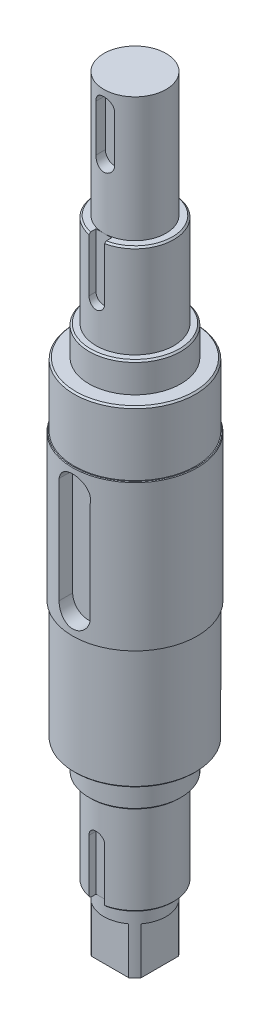
SolidWorks part; units mm, degrees
material "1045"
ref_plane "Front Plane" through (0, 0, 0) normal (0, 0, 1) x (1, 0, 0)
ref_plane "Top Plane" through (0, 0, 0) normal (0, 1, 0) x (1, 0, 0)
ref_plane "Right Plane" through (0, 0, 0) normal (1, 0, 0) x (0, 0, -1)
sketch "Sketch1" plane through (0, 0, 0) normal (0, 1, 0) x (1, 0, 0)
  circle A0 centre (0, 0) radius 20
  dimension "D1" = 40
extrude "Extrude1" add sketch "Sketch1" along normal blind 32 and the other way blind 15
sketch "草图1" plane through (0, -15, 0) normal (0, -1, 0) x (1, 0, 0)
  circle A0 centre (0, 0) radius 19.5
  dimension "D1" = 39
extrude "拉伸1" add sketch "草图1" along normal blind 38.5
sketch "Sketch2" plane through (0, 32, 0) normal (0, 1, 0) x (1, 0, 0)
  circle A0 centre (0, 0) radius 19.5
  dimension "D1" = 39
extrude "Extrude2" add sketch "Sketch2" along normal blind 20.5
ref_plane "Plane1" through (0, 0, 20) normal (0, 0, 1) x (1, 0, 0)
chamfer "Chamfer1" distance 0.2 angle 45 1 edges at (0, 32, 20)
sketch "Sketch4" plane through (0, 0, 20) normal (0, 0, 1) x (1, 0, 0)
  line L0 (0, 32) -> (0, -15) construction
  line L1 (19.8, 32) -> (-19.8, 32) construction
  line L2 (-19.5, -15) -> (19.5, -15) construction
  line L4 (-5, 26) -> (-5, -8)
  line L5 (5, 24) -> (5, -8)
  arc A0 (-5, 26) -> (5, 24) centre (0, 25) cw
  arc A1 (-5, -8) -> (5, -8) centre (0, -8) ccw
  dimension "D1" = 7
  dimension "D2" = 10
extrude "Cut-Extrude1" cut sketch "Sketch4" against normal blind 5
sketch "Sketch5" plane through (0, 52.5, 0) normal (0, 1, 0) x (1, 0, 0)
  circle A0 centre (0, 0) radius 14.75
  dimension "D1" = 29.5
extrude "Extrude3" add sketch "Sketch5" along normal blind 9.5
sketch "Sketch6" plane through (0, 62, 0) normal (0, 1, 0) x (1, 0, 0)
  circle A0 centre (0, 0) radius 12.5
  dimension "D1" = 25
extrude "Extrude4" add sketch "Sketch6" along normal blind 30
sketch "Sketch7" plane through (0, -53.5, 0) normal (0, -1, 0) x (1, 0, 0)
  circle A0 centre (0, 0) radius 14.75
  dimension "D1" = 29.5
extrude "Extrude5" add sketch "Sketch7" along normal blind 9.5
sketch "Sketch8" plane through (0, -63, 0) normal (0, -1, 0) x (1, 0, 0)
  circle A0 centre (0, 0) radius 12.5
  dimension "D1" = 25
extrude "Extrude6" add sketch "Sketch8" along normal blind 30
chamfer "Chamfer2" distance 0.5 angle 45 5 edges at (0, -53.5, -19.5) (0, -63, -14.75) (0, 52.5, 19.5) (0, 62, 14.75) (0, 92, 12.5)
sketch "Sketch9" plane through (0, 92, 0) normal (0, 1, 0) x (1, 0, 0)
  circle A0 centre (0, 0) radius 10
  dimension "D1" = 20
extrude "Extrude7" add sketch "Sketch9" along normal blind 40
ref_plane "Plane2" through (0, 0, 11) normal (0, 0, 1) x (1, 0, 0)
sketch "Sketch10" plane through (0, 0, 11) normal (0, 0, 1) x (1, 0, 0)
  line L0 (0, 132) -> (0, 92) construction
  line L1 (10, 132) -> (-10, 132) construction
  line L2 (12, 92) -> (-12, 92) construction
  line L5 (-3, 127) -> (-3, 112)
  line L7 (3, 127) -> (3, 112)
  arc A0 (-3, 112) -> (3, 112) centre (0, 112) ccw
  arc A1 (-3, 127) -> (3, 127) centre (0, 127) cw
  dimension "D1" = 20
  dimension "D2" = 5
  dimension "D3" = 6
extrude "Cut-Extrude2" cut sketch "Sketch10" against normal blind 4.5
sketch "Sketch11" plane through (0, -93, 0) normal (0, -1, 0) x (1, 0, 0)
  circle A0 centre (0, 0) radius 10
  dimension "D1" = 20
extrude "Boss-Extrude1" add sketch "Sketch11" along normal blind 20
sketch "Sketch12" plane through (0, -113, 0) normal (0, -1, 0) x (1, 0, 0)
  line L1 (-8, 8) -> (8, 8)
  line L2 (-8, 8) -> (-8, -8)
  line L3 (-8, -8) -> (8, -8)
  line L4 (8, 8) -> (8, -8)
  line L5 (-8, 8) -> (8, -8) construction
  line L6 (-8, -8) -> (8, 8) construction
  point P0 (0, 0)
  dimension "D1" = 16
  dimension "D2" = 16
extrude "Cut-Extrude3" cut sketch "Sketch12" against normal blind 15 flip side to cut
chamfer "Chamfer3" distance 0.5 angle 45 1 edges at (0, -93, -12.5)
ref_plane "Plane3" through (0, 0, 10) normal (0, 0, 1) x (1, 0, 0)
sketch "Sketch13" plane through (0, 0, 10) normal (0, 0, 1) x (1, 0, 0)
  line L0 (0, 92) -> (0, 74.5) construction
  line L1 (12, 92) -> (-12, 92) construction
  line L2 (2.5, 92) -> (2.5, 74.5)
  line L3 (-2.5, 92) -> (-2.5, 74.5)
  line L4 (0, -93) -> (0, -75.5) construction
  line L5 (-10, -93) -> (10, -93) construction
  line L6 (-2.5, -93) -> (-2.5, -75.5)
  line L7 (2.5, -93) -> (2.5, -75.5)
  arc A0 (2.5, 92) -> (-2.5, 92) centre (0, 92) ccw
  arc A1 (-2.5, 74.5) -> (2.5, 74.5) centre (0, 74.5) ccw
  arc A2 (-2.5, -93) -> (2.5, -93) centre (0, -93) ccw
  arc A3 (2.5, -75.5) -> (-2.5, -75.5) centre (0, -75.5) ccw
  point P5 (0, 83.25)
  point P14 (0, -84.25)
  dimension "D1" = 5
  dimension "D2" = 17.5
  dimension "D3" = 5
  dimension "D4" = 17.5
extrude "Cut-Extrude4" cut sketch "Sketch13" along normal blind 10
